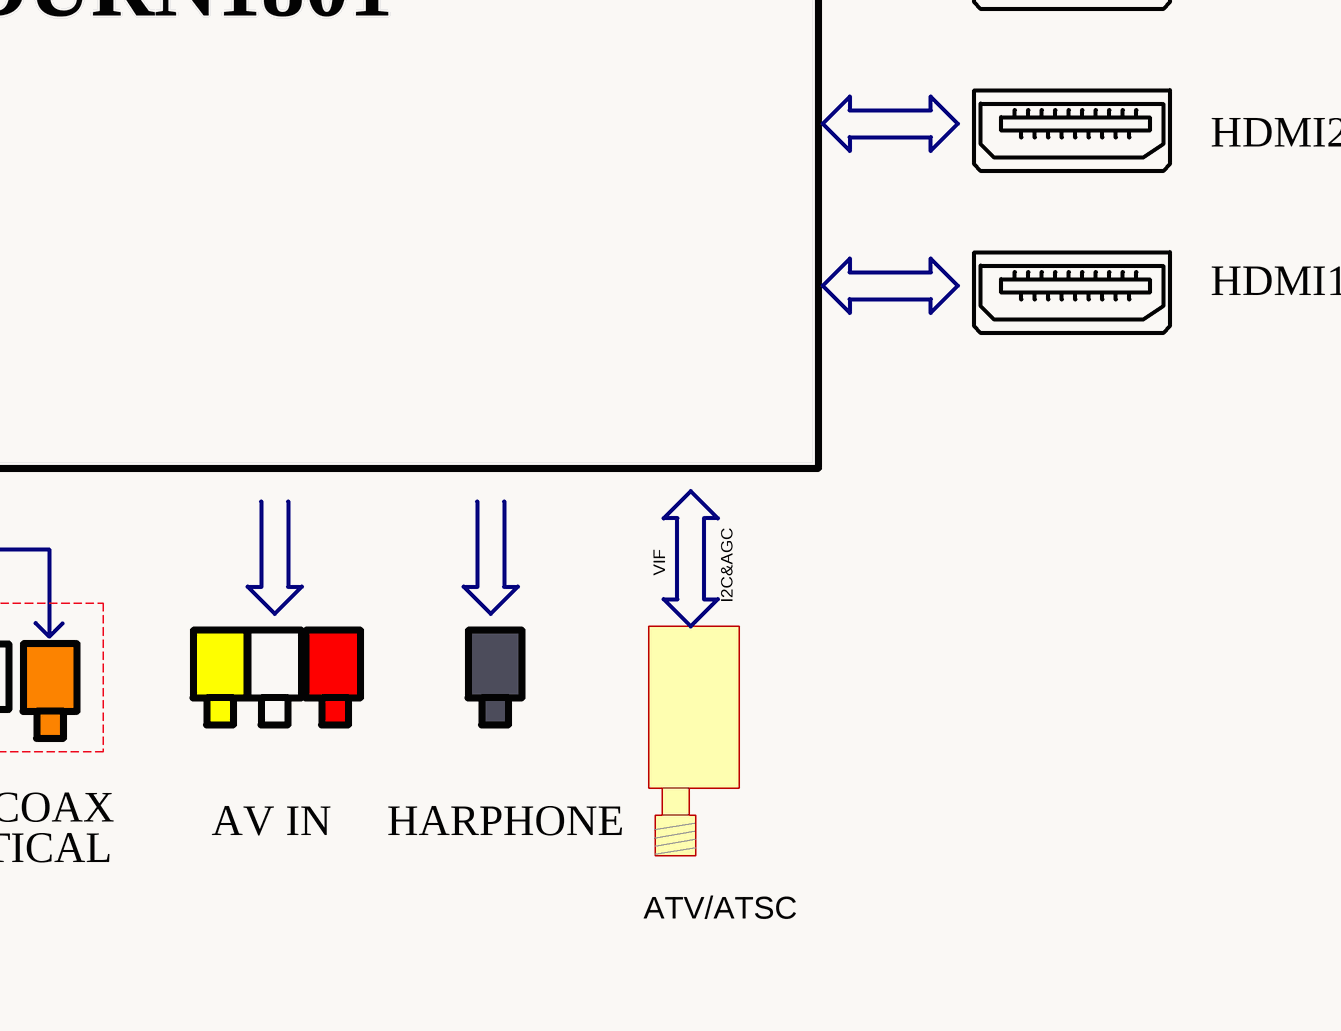
[diagram p0: MISC86290-5.SchDoc, bottom right]
# Altium project MISC86290.PrjPcb (part 3 of 13)

## Sheet MISC86290-5.SchDoc (continued)

### Parts
(Parts that share a designator on the sheet are numbered #1, #2 ... from top to bottom, then left to right.)
*  JAE connector  (value not drawn)
AMP  Name: AMP_2.0(2*15W/8Ω)  (hidden comment: AMP)  (graphical)
AV_IN  AV IN  (graphical)
COAX#1  Name: *COAX  (hidden comment: COAX)  (graphical)
EARPHONE#1  Name: LINEOUT  (hidden comment: EARPHONE)  (graphical)
EARPHONE#2  Name: HARPHONE  (hidden comment: EARPHONE)  (graphical)
HDMI#1  Name: HDMI1  (hidden comment: HDMI)  (graphical)
HDMI#2  Name: HDMI2  (hidden comment: HDMI)  (graphical)
HDMI#3  Name: HDMI3  (hidden comment: HDMI)  (graphical)
HDMI#4  Name: HDMI4  (hidden comment: HDMI)  (graphical)
IR&KEY  IR&KEY  (value not drawn)
MAINBOARD  MAINBOARD  (value not drawn)
OPTICAL#1  OPTICAL  (graphical)
RJ45  RJ45  (graphical)
USB0/USB1  USB0/USB1  (graphical)

### Notes on the sheet
- Main Board Power Tree
- SYSTEM FUNCTION BLOCK DIAGRAM
- UA2
- 70mA
- HEADPHONE AMP
- AD22653B
- INVERTER
- EXT_WIFI
- UA3
- LINEOUT AMP
- U1
- QM1
- UL2
- MSDURN1801
- MOSFET
- 3V3_M
- 540mA
- LDO
- 100mA
- MOD_1V2
- AO3487
- LC1117CLTR12
- 300mA
- UD2
- 2400mA
- UD3
- AVDD/VDDP
- 800mA
- DC-DC
- 3V3_STB
- 850mA
- DC/DC
- 1000mA
- 1V5_DDR
- VCC_DDR
- VB1
- TPS563201
- TLV62569PDDC
- 350mA
- AVDD33
- 3V3_WIFI
- WIFI
- *
- 12V
- UD1
- 2435mA
- 5V_M
- UD5
- 0.95V_VDDCPU
- PSU
- 3650mA
- 1200mA
- TPS564201
- 1185mA
- 335mA
- 1500mA
- UD4
- 0.95V_VDDC
- AMP_VCC(24V)
- TLV62095RGTR
- 3800mA
- UH3
- SWITCH
- USB_5V
- USB1
- APL3551CBI-TRG
- USB2
- UL1
- 250mA
- 3V3_Tun
- UT2
- LC1117CLTR33
- TUNER
- SI2151
- VIF
- I2C&AGC
- QM2
- PANEL
- VCC_Panel
- AO4459
- UA1
- AMP
- TAS5751
- ATV/ATSC

### Library data of the parts
AMP = AMP_2.0(2*8W/8Ω)
MAINBOARD = IR&KEY
AV_IN = AV IN: Name: AV IN
OPTICAL#1 = OPTICAL: Name: OPTICAL
RJ45 = RJ45: Name: RJ45
USB0/USB1 = USB0/USB1: Name: USB0/USB1